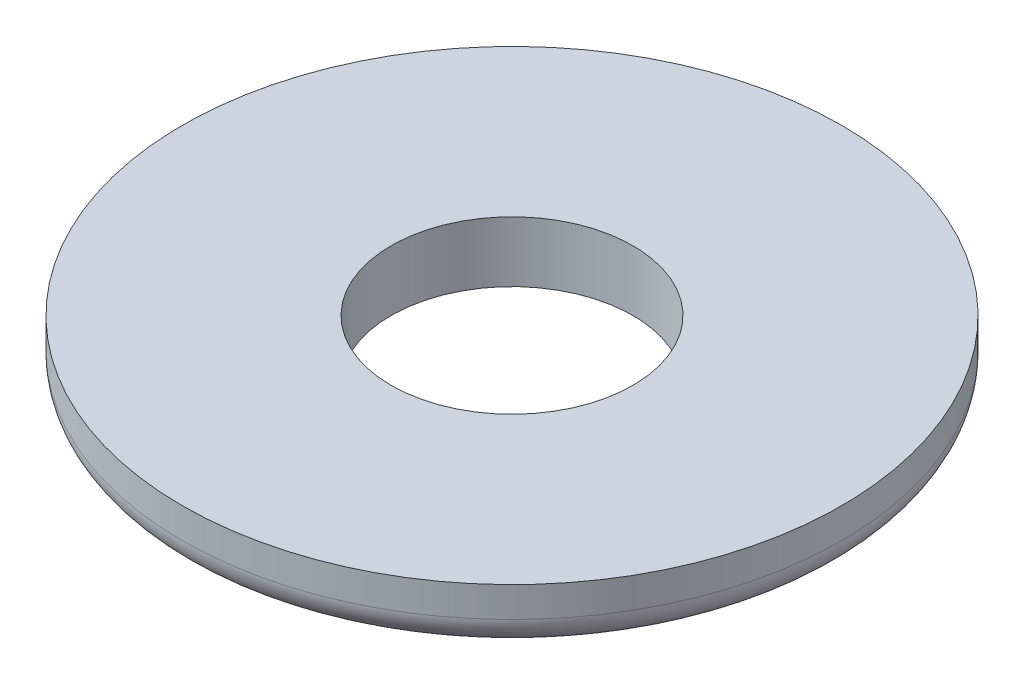
SolidWorks part; units mm, degrees
ref_plane "前视基准面" through (0, 0, 0) normal (0, 0, 1) x (1, 0, 0)
ref_plane "上视基准面" through (0, 0, 0) normal (0, 1, 0) x (1, 0, 0)
ref_plane "右视基准面" through (0, 0, 0) normal (1, 0, 0) x (0, 0, -1)
sketch "草图1" plane through (0, 0, 0) normal (0, 0, 1) x (1, 0, 0)
  line L0 (0, 51.8209) -> (0, -36.1036) construction
  line L1 (20, 2.953) -> (20, -7.047)
  line L2 (20, -7.047) -> (49.5, -7.047)
  line L3 (54.5, -2.047) -> (54.5, 2.953)
  line L4 (54.5, 2.953) -> (20, 2.953)
  line L5 (20, 2.953) -> (20.3774, 4.085)
  arc A0 (49.5, -7.047) -> (54.5, -2.047) centre (49.5, -2.047) ccw
  dimension "D4" = 5
  dimension "D1" = 20
  dimension "D2" = 10
  dimension "D3" = 34.5
revolve "旋转1" add sketch "草图1" angle 360 about L0
